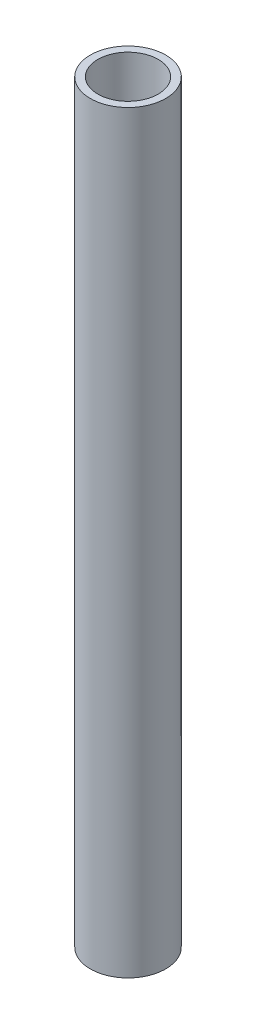
from build123d import *

# Parameters (mm, degrees)
SKETCH11_R                             = 10
SKETCH11_R_2                           = 8
GB_T_6728_2002_ROUND_TUBE_20_2_1_DEPTH = 200


with BuildPart() as part:
    # Sketch11 → GB/T 6728-2002 round tube 20 × 2(1) (new body)
    with BuildSketch(Plane(origin=(0, 0, 0), x_dir=(-1, 0, 0), z_dir=(0, 1, 0))):
        Circle(SKETCH11_R)
        Circle(SKETCH11_R_2, mode=Mode.SUBTRACT)
    extrude(amount=GB_T_6728_2002_ROUND_TUBE_20_2_1_DEPTH)


solid = part.part
